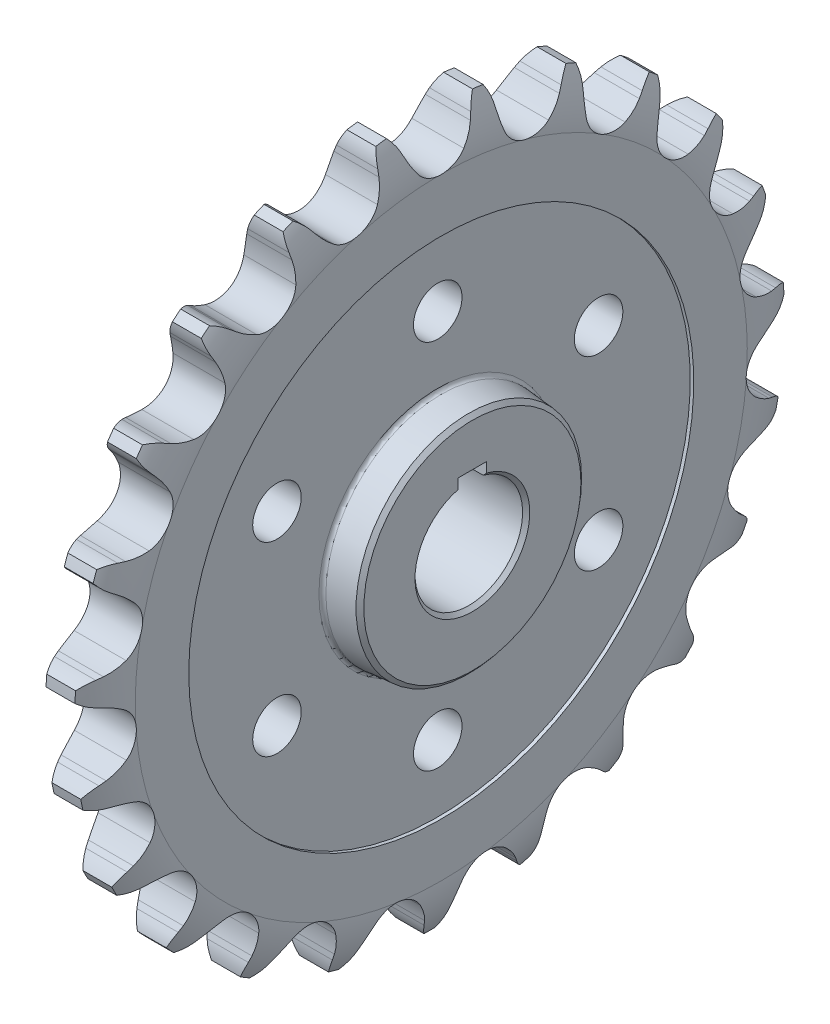
SolidWorks part; units mm, degrees
ref_plane "前视基准面" through (0, 0, 0) normal (0, 0, 1) x (1, 0, 0)
ref_plane "上视基准面" through (0, 0, 0) normal (0, 1, 0) x (1, 0, 0)
ref_plane "右视基准面" through (0, 0, 0) normal (1, 0, 0) x (0, 0, -1)
sketch "草图1" plane through (0, 0, 0) normal (0, 0, 1) x (1, 0, 0)
  line L0 (-12.7, 0) -> (12.7, 0) construction
  line L1 (-6.35, 15) -> (-6.35, 70.4081)
  line L2 (-6.35, 70.4081) -> (-7.3238, 70.4081)
  line L3 (-7.3238, 70.4081) -> (-7.3238, 85.3281)
  line L4 (-4.0218, 99) -> (4.0218, 99)
  line L5 (7.3238, 85.3281) -> (7.3238, 70.4081)
  line L6 (7.3238, 70.4081) -> (6.35, 70.4081)
  line L7 (6.35, 70.4081) -> (6.35, 15)
  line L8 (6.35, 15) -> (-6.35, 15)
  line L9 (0, 0) -> (0, 99) construction
  line L10 (-6.4112, 93.2681) -> (6.4112, 93.2681) construction
  line L11 (-6.4112, -93.2681) -> (6.4112, -93.2681) construction
  line L12 (12.7, 0) -> (35.7, 0) construction
  line L13 (-7.3238, 85.3281) -> (3.7984, 85.3281) construction
  line L14 (-7.3238, -85.3281) -> (3.7984, -85.3281) construction
  line L15 (35.7, 0) -> (51.58, 0) construction
  line L16 (51.58, 0) -> (75.71, 0) construction
  line L17 (75.71, 0) -> (91.46, 0) construction
  line L18 (91.46, 0) -> (120.75, 0) construction
  arc A0 (-4.0218, 99) -> (-7.3238, 85.3281) centre (18.0522, 86.4341) ccw
  arc A1 (4.0218, 99) -> (7.3238, 85.3281) centre (-18.0522, 86.4341) cw
  point P30 (7.3238, 70.4081)
  point P33 (-7.3238, 70.4081)
  dimension "rx" = 25.4
  dimension "d" = 186.5361
  dimension "p" = 25.4
  dimension "z" = 23
  dimension "da" = 198
  dimension "df" = 170.6561
  dimension "dr" = 15.88
  dimension "dk" = 30
  dimension "h" = 24.13
  dimension "bf1" = 14.6475
  dimension "b1" = 15.75
  dimension "ba" = 3.302
  dimension "pt" = 29.29
  dimension "t" = 12.7
  dimension "C2" = 22.86
revolve "旋转1" add sketch "草图1" angle 360 about L0
sketch "草图2" plane through (0, 0, 0) normal (1, 0, 0) x (0, 0, -1)
  line L0 (0, 0) -> (0, 99) construction
  line L1 (0, 0) -> (-13.4805, 98.0779) construction
  line L2 (0, 0) -> (-26.7099, 95.3288) construction
  line L3 (6.3611, 88.3678) -> (25.8446, 73.3588) construction
  line L4 (9.154, 93.2393) -> (-10.0641, 101.0209) construction
  line L5 (0, 0) -> (13.4805, 98.0779) construction
  line L6 (9.154, 93.2393) -> (9.7775, 94.7791)
  line L7 (-9.154, 93.2393) -> (-9.7775, 94.7791)
  circle A0 centre (0, 0) radius 99 construction
  arc A1 (6.3611, 88.3678) -> (-6.3611, 88.3678) centre (0, 93.2681) cw
  arc A2 (6.3611, 88.3678) -> (9.154, 93.2393) centre (-10.0641, 101.0209) ccw
  arc A3 (11.9923, 98.271) -> (9.7775, 94.7791) centre (20.4517, 90.457) ccw
  arc A4 (-6.3611, 88.3678) -> (-9.154, 93.2393) centre (10.0641, 101.0209) cw
  arc A5 (-11.9923, 98.271) -> (-9.7775, 94.7791) centre (-20.4517, 90.457) cw
  arc A7 (11.9923, 98.271) -> (-11.9923, 98.271) centre (0, 0) ccw
  dimension "r1" = 8.0297
  dimension "r3" = 11.5161
  dimension "D1" = 15.652
  dimension "D2" = 7.826
  dimension "α/2" = 52.391
  dimension "M" = 10.0641
  dimension "T" = 7.7528
  dimension "β" = 15.565
  dimension "γ/2" = 14.217
  dimension "bc" = 1.6613
extrude "切除-拉伸1" cut sketch "草图2" against normal mid plane 21.9712
pattern_circular "阵列(圆周)1" count 23 over 360 about axis through (0, 0, 0) along (1, 0, 0) of "切除-拉伸1"
sketch "草图4" plane through (-6.35, 0, 0) normal (-1, 0, 0) x (0, 0, 1)
  line L1 (-4, 14.4568) -> (4, 14.4568)
  line L2 (-4, 14.4568) -> (-4, 18.3)
  line L3 (-4, 18.3) -> (4, 18.3)
  line L4 (4, 14.4568) -> (4, 18.3)
  circle A0 centre (0, 0) radius 15 construction
  point P6 (0.7, 18.3)
  dimension "D1" = 18.3
  dimension "键槽宽度" = 8
  dimension "t1" = 3.3
sketch "草图5" plane through (0, 0, 0) normal (0, 0, 1) x (1, 0, 0)
  line L1 (-16, 15) -> (16, 15)
  line L2 (-16, 15) -> (-16, 31.3654)
  line L3 (-16, 31.3654) -> (-6.35, 32.2096)
  line L4 (16, 15) -> (16, 31.3654)
  line L6 (0, 0) -> (0, -4.2677) construction
  line L7 (0, 0) -> (-10.4728, 0) construction
  line L8 (-6.35, 15) -> (-6.35, 70.4081) construction
  line L9 (-6.35, 32.2096) -> (6.35, 32.2096)
  line L10 (6.35, 70.4081) -> (6.35, 15) construction
  line L11 (6.35, 32.2096) -> (16, 31.3654)
  dimension "D1" = 5
  dimension "L" = 32
  dimension "H" = 16.3654
revolve "旋转2" add sketch "草图5" angle 360 about L7
extrude "切除-拉伸2" cut sketch "草图4" against normal through all
mirror "镜向1" about plane through (0, 0, 0) normal (1, 0, 0) of "切除-拉伸2"
fillet "圆角1" radius 1.016 2 edges at (6.35, 0, -32.2096) (-6.35, 0, -32.2096)
chamfer "倒角1" distance 1 angle 45 4 edges at (16, -15, 0) (16, 0, -31.3654) (-16, -15, 0) (-16, 0, -31.3654)
sketch "草图6" plane through (-6.35, 0, 0) normal (-1, 0, 0) x (0, 0, 1)
  line L0 (0, 70.4081) -> (0, 45.0081) construction
  line L1 (0, 45.0081) -> (0, 58.5406) construction
  line L2 (0, 58.5406) -> (0, 33.1406) construction
  line L3 (0, 33.1406) -> (0, 0) construction
  circle A0 centre (0, 51.7743) radius 6.7663
  circle A1 centre (0, 0) radius 70.4081 construction
  circle A2 centre (0, 0) radius 70.4081 construction
  circle A3 centre (0, 0) radius 33.1406 construction
  dimension "g" = 25.4
extrude "切除-拉伸3" cut sketch "草图6" against normal through all
pattern_circular "阵列(圆周)2" count 6 over 360 about axis through (0, 0, 0) along (1, 0, 0) of "切除-拉伸3"
